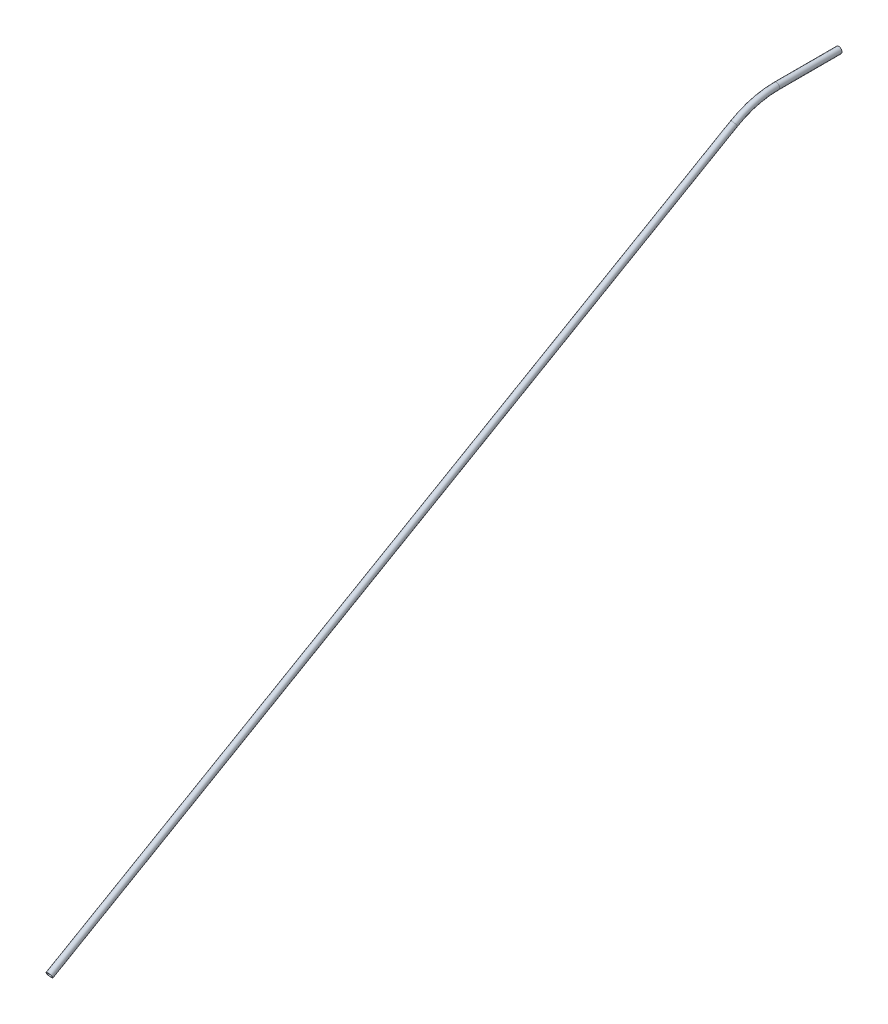
from build123d import *

# Parameters (mm, degrees)
SKETCH1_R   = 11
SKETCH1_R_2 = 9


with BuildPart() as part:
    # Sweep1: sweep along a path in Sketch2
    with BuildLine(Plane(origin=(0, 0, 0), x_dir=(0, 0, -1), z_dir=(1, 0, 0))) as sweep1_path:
        Line((0, 0), (-219.615242271, 0))
        ThreePointArc((-219.615242271, 0), (-297.260955801, -10.222252113), (-369.615242271, -40.192378865))
        Line((-369.615242271, -40.192378865), (-2780.296756439, -1432))
    # Sketch1 → Sweep1 (sweep)
    with BuildSketch(Plane.XY):
        Circle(SKETCH1_R)
        Circle(SKETCH1_R_2, mode=Mode.SUBTRACT)
    sweep(path=sweep1_path.line)


solid = part.part
